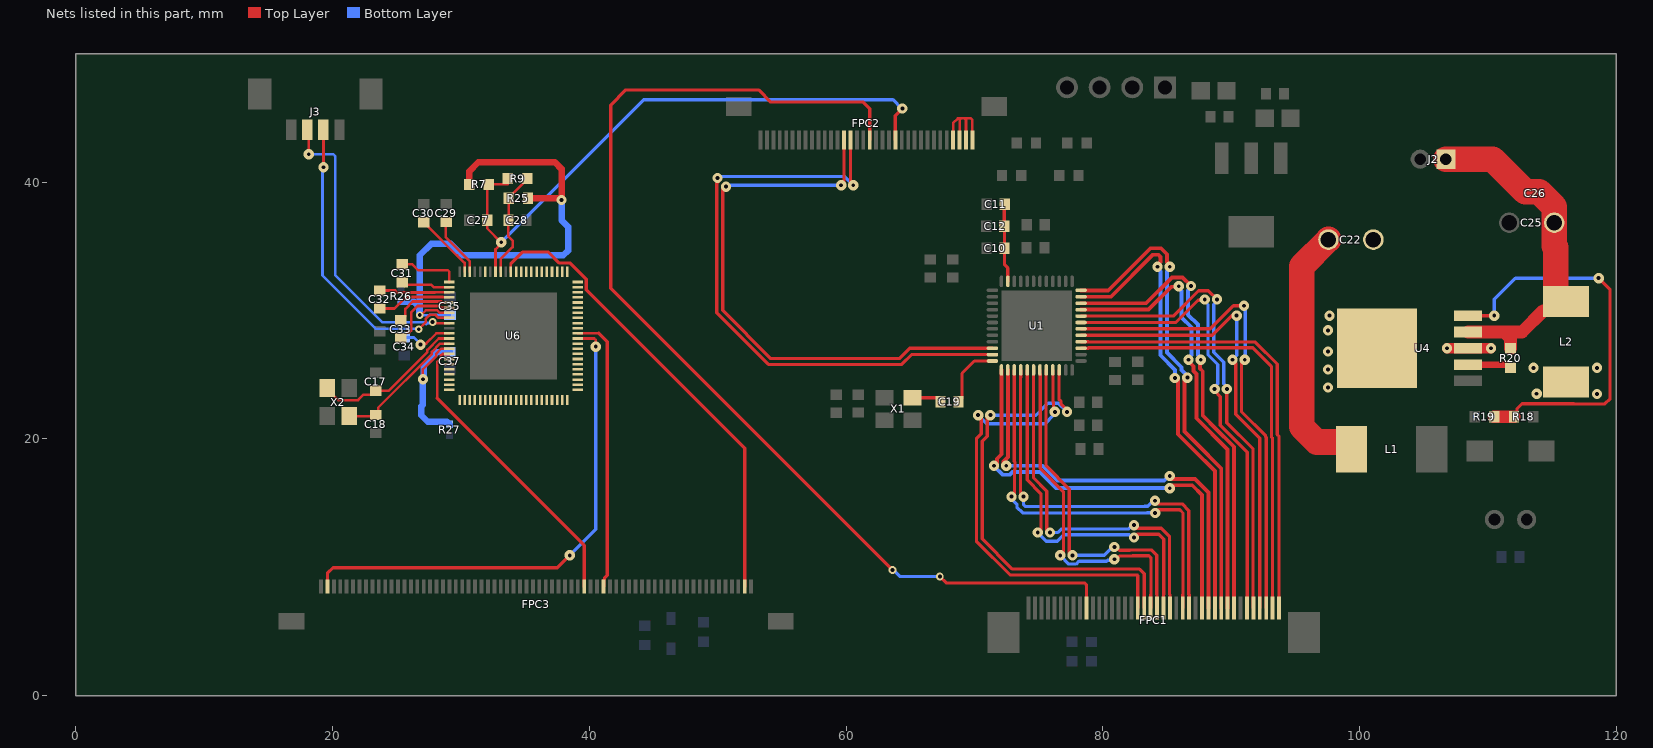
[diagram p0: the nets of this part, all layers, seen from the top]
# Altium PCB MISC71201-3.PcbDoc (part 3 of 3)
Units mm, origin at the board's own origin, x right, y up, seen from the top; angles counter-clockwise.
Board outline 120 x 50 mm, 4 copper layers (Top Layer, Layer 1, Layer 2, Bottom Layer), stack 0.603 mm thick; 69 components, 139 nets, 430 pads, 271 vias.

## Via types
v1: diameter 0.8, hole 0.3, Top Layer to Bottom Layer, 182 vias
v2: diameter 0.6, hole 0.3, Top Layer to Bottom Layer, 89 vias

## Nets (pads, with @x,y where several pads share a name; then routed paths per layer and width w, separated by ;. In a path a pad name is that pad's centre, name@x,y a point inside that pad or via, vN(x,y) a via of type N, cw(c..) or ccw(c..) an arc to the next point about the centre after c; other vN are vias at no path point) (continued)
MIPI_TD3_N: FPC2.15 U1.23 | length 48.6
  Top Layer w0.254: v1(49.986,40.311) 50.098,40.199 50.098,40.072 49.943,39.917 49.943,29.809 53.956,25.796 64.337,25.796 65.102,26.561 U1.23@71.407,26.561 ; FPC2.15@60.345,43.277 60.344,42.4 60.344,39.976 v1(60.57,39.751)
  Bottom Layer w0.254: v1(49.986,40.311) 50.103,40.428 59.9,40.428 60.57,39.758 v1(60.57,39.751)
MIPI_TD3_P: FPC2.14 U1.22 | length 45.6
  Top Layer w0.254: v1(50.658,39.639) 50.546,39.751 50.419,39.751 50.397,39.729 50.397,29.997 54.144,26.25 64.149,26.25 64.961,27.061 U1.22@71.407,27.061 ; v1(59.62,39.751) 59.844,39.975 59.844,42.4 FPC2.14@59.845,43.277
  Bottom Layer w0.254: v1(50.658,39.639) 50.77,39.751 v1(59.62,39.751)
NetC10_2: C10.2 C11.2 C12.1 U1.11 | length 6.2
  Top Layer w0.254: C11.2@72.367,38.28 72.319,38.232 C12.1@72.319,36.546 72.337,36.528 C10.2@72.337,34.851 72.337,33.581 72.606,33.312 U1.11@72.606,32.261
NetC19_1: C19.1 U1.24 | length 5.1
  Top Layer w0.254: C19.1@68.763,22.893 69.036,23.166 69.036,25.094 70.003,26.061 U1.24@71.407,26.061
NetC19_2: C19.2 X1.3 | length 2.3
  Top Layer w0.254: X1.3@65.184,23.208 67.09,23.208 67.363,22.935 C19.2@67.363,22.893
NetC22_1: C22.1 L2.1 U4.3 U4.6 | length 3.4
  Top Layer w0.8: v1(106.807,27.051) U4.3@108.445,27.051 v1(110.236,27.051)
  other v1: 118.491,23.495 113.792,23.514 97.536,24.003 97.536,25.4 113.538,25.527 118.491,25.527 97.536,26.797 97.536,28.448 97.663,29.591
NetC22_2: C22.2 L1.1 | length 20.2
  Top Layer w2: C22.2@97.575,35.519 95.504,33.448 95.504,20.928 96.676,19.756 99.149,19.756 99.361,19.544 L1.1@99.361,19.177
NetC31_1: C31.1 U6.1 | length 4.7
  Top Layer w0.2: C31.1@25.446,33.599 26.208,33.599 26.678,33.129 28.984,33.129 29.101,33.012 U6.1@29.101,32.215
NetC31_2: C31.2 U6.2 | length 3.8
  Top Layer w0.2: C31.2@25.446,32.2 25.641,32.004 27.686,32.004 27.875,31.815 U6.2@29.101,31.815
NetC32_1: C32.1 U6.3 | length 5.5
  Top Layer w0.2: C32.1@23.675,31.552 24.89,31.552 25.045,31.397 27.968,31.397 27.986,31.415 U6.3@29.101,31.415
NetC32_2: C32.2 U6.4 | length 5.8
  Top Layer w0.2: C32.2@23.675,30.152 24.818,30.152 25.713,31.047 28.612,31.047 28.644,31.015 U6.4@29.101,31.015
NetC33_1: C33.1 U6.5 | length 4.7
  Top Layer w0.2: C33.1@25.326,29.251 25.376,29.251 25.676,29.551 25.676,30.121 26.252,30.697 28.467,30.697 28.549,30.615 U6.5@29.101,30.615
NetC33_2: C33.2 U6.6 | length 5.7
  Top Layer w0.2: C33.2@25.326,27.851 25.376,27.851 25.829,28.304 26.006,28.304 26.147,28.446 26.147,29.86 26.634,30.347 28.322,30.347 28.454,30.215 U6.6@29.101,30.215
NetR18_1: R18.1 R19.1 U4.5 | length 31.7
  Top Layer w0.254: U4.5@108.445,29.591 v1(110.49,29.591) ; R18.1@112.024,21.717 112.262,21.955 112.262,22.346 112.649,22.733 116.675,22.733 116.694,22.714 119.107,22.714 119.507,23.114 119.507,31.623 v1(118.618,32.512)
  Top Layer w1: R19.1@110.48,21.717 R18.1@112.024,21.717
  Bottom Layer w0.254: v1(110.49,29.591) 110.49,30.861 112.141,32.512 v1(118.618,32.512)
NetR20_1: R20.1 U4.2 | length 3.4
  Top Layer w0.254: R20.1@111.516,25.781 R20.1@111.76,25.537
  Top Layer w0.5: U4.2@108.445,25.781 R20.1@111.516,25.781
PWM: FPC1.10 FPC2.18 | length 86.4
  Top Layer w0.254: FPC2.18@61.845,43.277 61.845,45.724 61.341,46.228 54.133,46.228 53.189,47.173 42.855,47.173 41.67,45.988 41.67,31.736 v2(63.627,9.779) ; v2(67.31,9.271) 67.804,8.777 78.577,8.777 78.726,8.628 FPC1.10@78.726,6.825
  Bottom Layer w0.254: v2(63.627,9.779) 63.706,9.779 64.214,9.271 v2(67.31,9.271)
RESET#: C27.1 FPC2.22 R7.1 R9.2 U6.81 | length 48.2
  Top Layer w0.2: U6.81@32.701,33.015 32.701,34.762 33.147,35.208 v1(33.147,35.306) 32.06,36.393 C27.1@32.06,37.031 32.06,39.707 R7.1@32.171,39.818 33.663,39.818 R9.2@33.663,40.259
  Top Layer w0.254: FPC2.22@63.845,43.277 63.845,45.16 64.389,45.704 v1(64.389,45.72)
  Bottom Layer w0.254: v1(33.147,35.306) 44.243,46.402 63.666,46.402 64.348,45.72 v1(64.389,45.72)
RFU_NC: FPC2.31 FPC2.32 FPC2.33 FPC2.34 | length 8
  Top Layer w0.2: FPC2.31@68.345,43.277 68.345,44.596 68.707,44.958 68.962,44.958 ; FPC2.32@68.845,43.277 68.845,44.841 68.962,44.958 ; FPC2.33@69.345,43.277 69.345,44.83 69.217,44.958 ; FPC2.34@69.845,43.277 69.845,44.841 69.728,44.958 69.217,44.958 ; 68.962,44.958 69.217,44.958
RX1: FPC3.42 U6.15 | length 23.6
  Top Layer w0.21: 28.154,23.154 28.154,25.995 28.446,26.287 28.446,26.487 28.569,26.61 29.096,26.61 U6.15@29.101,26.615
  Top Layer w0.254: 28.154,23.154 39.61,11.698 FPC3.42@39.61,8.484
RX2: U6.16
RX3: U6.17
RX4: U6.18
RX5: U6.19
RX6: U6.20
RX7: U6.21
RX8: U6.22
RX9: U6.23
RX10: U6.24
RX11: U6.25
RX12: U6.26
RX13: U6.27
RX14: U6.28
RX15: U6.29
RX16: U6.30
RX17: U6.31
RX18: U6.32
RX19: U6.33
RX20: U6.34
RX21: U6.35
RX22: U6.36
RX23: U6.37
RX24: U6.38
RX25: U6.39
RX26: U6.40
RX27: U6.41
RX28: U6.42
RX29: U6.43
RX30: U6.44
RX31: U6.45
RX32: U6.46
RX33: U6.47
RX34: U6.48
RX35: U6.49
RX36: U6.50
RX37: U6.51
RX38: U6.52
RX39: U6.53
RX40: U6.54
RX41: FPC3.2 U6.55 | length 39.6
  Top Layer w0.2: U6.55@39.101,27.815 40.384,27.815 40.513,27.686 v1(40.513,27.178)
  Top Layer w0.254: FPC3.2@19.61,8.484 19.61,9.525 20.043,9.958 37.517,9.958 v1(38.481,10.922)
  Bottom Layer w0.254: v1(38.481,10.922) 40.513,12.954 v1(40.513,27.178)
RXE0_N: FPC1.30 U1.47 | length 36.9
  Top Layer w0.3: U1.47@78.306,31.062 80.633,31.062 83.913,34.342 84.316,34.342 84.492,34.166 84.492,33.761 84.267,33.536 v1(84.267,33.401) ; v1(85.615,24.745) 85.655,24.745 85.86,24.54 85.86,20.359 87.042,19.177 88.726,17.493 88.726,7.875 FPC1.30@88.726,6.825
  Bottom Layer w0.3: v1(84.267,33.401) 84.267,33.266 84.492,33.041 84.492,26.504 85.632,25.364 85.632,24.762 v1(85.615,24.745)
RXE0_P: FPC1.31 U1.48 | length 37.9
  Top Layer w0.3: U1.48@78.306,31.562 80.426,31.562 83.706,34.842 84.523,34.842 84.992,34.373 84.992,33.761 85.217,33.536 v1(85.217,33.401) ; v1(86.585,24.765) 86.36,24.54 86.36,20.566 87.249,19.677 89.226,17.7 89.226,7.875 FPC1.31@89.226,6.825
  Bottom Layer w0.3: v1(85.217,33.401) 85.217,33.266 84.992,33.041 84.992,26.712 86.132,25.571 86.132,25.353 86.585,24.9 v1(86.585,24.765)
RXE1_N: FPC1.32 U1.45 | length 35.2
  Top Layer w0.3: U1.45@78.306,30.061 83.574,30.061 85.353,31.84 85.881,31.84 v1(85.918,31.877) ; v1(86.68,26.162) 86.68,26.027 87.059,25.648 87.059,25.281 87.285,25.055 87.285,21.607 89.726,19.166 FPC1.32@89.726,6.825
  Bottom Layer w0.3: v1(85.918,31.877) 85.918,31.742 86.143,31.517 86.143,29.451 86.905,28.689 86.905,26.522 86.68,26.297 v1(86.68,26.162)
RXE1_P: FPC1.33 U1.46 | length 36.4
  Top Layer w0.3: U1.46@78.306,30.562 83.367,30.561 85.383,32.577 86.208,32.577 86.868,31.917 v1(86.868,31.907) ; v1(87.63,26.162) 87.559,26.091 87.559,25.488 87.785,25.262 87.785,21.814 88.9,20.699 90.079,19.52 90.226,19.373 FPC1.33@90.226,6.825
  Bottom Layer w0.3: v1(86.868,31.907) 86.868,31.771 86.643,31.546 86.643,29.658 87.405,28.896 87.405,26.522 87.63,26.297 v1(87.63,26.162)
RXE2_N: FPC1.35 U1.43 | length 36
  Top Layer w0.254: U1.43@78.306,29.06 85.687,29.06 87.417,30.79 87.879,30.79 v1(87.946,30.857) ; v1(88.712,23.876) 88.712,23.728 89.154,23.286 89.154,21.049 91.249,18.954 91.249,6.848 FPC1.35@91.226,6.825
  Bottom Layer w0.254: v1(87.946,30.857) 87.946,30.71 88.196,30.46 88.196,26.553 88.96,25.789 88.96,24.272 88.712,24.024 v1(88.712,23.876)
RXE2_P: FPC1.36 U1.44 | length 37.1
  Top Layer w0.254: U1.44@78.306,29.561 85.48,29.561 87.453,31.534 88.227,31.534 v1(88.9,30.861) ; v1(89.662,23.876) 89.662,21.248 91.703,19.207 91.703,6.848 FPC1.36@91.726,6.825
  Bottom Layer w0.254: v1(88.9,30.861) 88.9,30.713 88.65,30.463 88.65,26.741 89.414,25.977 89.414,24.272 89.662,24.024 v1(89.662,23.876)
RXE3_N: FPC1.39 U1.39 | length 34.3
  Top Layer w0.254: U1.39@78.306,27.061 78.883,27.061 78.906,27.085 91.694,27.085 93.138,25.641 93.138,20.143 93.226,20.055 FPC1.39@93.226,6.825
RXE3_P: FPC1.40 U1.40 | length 35.1
  Top Layer w0.254: U1.40@78.306,27.562 78.883,27.562 78.906,27.539 91.882,27.539 93.592,25.829 93.592,20.331 93.726,20.197 FPC1.40@93.726,6.825
RXEC_N: FPC1.37 U1.41 | length 36.7
  Top Layer w0.254: U1.41@78.306,28.062 88.521,28.062 90.237,29.778 v1(90.424,29.591) ; v1(90.103,26.162) 90.351,25.914 90.351,21.917 92.226,20.042 FPC1.37@92.226,6.825
  Bottom Layer w0.254: v1(90.103,26.162) 90.103,26.169 90.424,26.49 v1(90.424,29.591)
RXEC_P: FPC1.38 U1.42 | length 37.9
  Top Layer w0.254: U1.42@78.306,28.563 88.38,28.563 90.175,30.358 v1(91,30.358) ; v1(91.053,26.162) 90.805,25.914 90.805,22.105 92.68,20.23 92.68,20.153 92.726,20.107 FPC1.38@92.726,6.825
  Bottom Layer w0.254: v1(91,30.358) 91.101,30.258 91.101,26.21 v1(91.053,26.162)
RXO0_N: FPC1.18 U1.33 | length 36.4
  Top Layer w0.254: v1(70.291,21.844) 70.412,21.844 70.539,21.717 70.539,20.381 70.158,20 70.158,12.012 72.772,9.398 82.677,9.398 82.726,9.349 FPC1.18@82.726,6.825 ; U1.33@76.106,25.362 76.106,25.045 76.13,25.022 76.13,22.89 76.162,22.858 76.162,22.202 v1(76.266,22.098)
  Bottom Layer w0.254: v1(70.291,21.844) 70.291,21.837 70.961,21.167 75.523,21.167 75.802,21.446 75.802,21.487 76.266,21.95 v1(76.266,22.098)
RXO0_P: FPC1.19 U1.34 | length 36.6
  Top Layer w0.254: v1(71.241,21.844) 71.12,21.844 70.993,21.717 70.993,20.193 70.612,19.812 70.612,12.2 72.96,9.852 82.865,9.852 83.226,9.491 FPC1.19@83.226,6.825 ; U1.34@76.607,25.362 76.607,25.045 76.584,25.022 76.584,23.078 76.752,22.909 76.752,22.709 77.216,22.246 v1(77.216,22.098)
  Bottom Layer w0.254: v1(71.241,21.844) 74.797,21.844 75.728,22.775 76.546,22.775 77.216,22.105 v1(77.216,22.098)
RXO1_N: FPC1.20 U1.31 | length 26.9
  Top Layer w0.254: U1.31@75.106,25.362 75.106,25.045 75.129,25.022 75.129,17.701 76.935,15.895 76.935,11.106 76.751,10.922 v1(76.687,10.922) ; v1(80.899,10.619) 81.047,10.619 81.295,10.867 82.292,10.867 82.317,10.892 83.6,10.892 83.749,10.743 83.749,7.875 83.726,7.852 FPC1.20@83.726,6.825
  Bottom Layer w0.254: v1(76.687,10.922) 76.687,10.915 77.357,10.245 77.918,10.245 78.141,10.468 80.292,10.468 80.373,10.549 80.829,10.549 v1(80.899,10.619)
RXO1_P: FPC1.21 U1.32 | length 26.6
  Top Layer w0.254: U1.32@75.606,25.362 75.606,25.045 75.583,25.022 75.583,17.889 77.389,16.083 77.389,11.106 77.573,10.922 v1(77.637,10.922) ; v1(80.899,11.569) 81.047,11.569 81.295,11.321 82.104,11.321 82.129,11.346 83.788,11.346 84.203,10.931 84.203,7.875 84.226,7.852 FPC1.21@84.226,6.825
  Bottom Layer w0.254: v1(77.637,10.922) 80.104,10.922 80.751,11.569 v1(80.899,11.569)
RXO2_N: FPC1.22 U1.29 | length 29.3
  Top Layer w0.254: U1.29@74.107,25.362 74.107,16.808 75.184,15.732 75.184,12.827 75.057,12.7 v1(74.936,12.7) ; v1(82.427,12.321) 82.427,12.329 82.671,12.573 84.368,12.573 84.749,12.192 84.749,7.875 84.726,7.852 FPC1.22@84.726,6.825
  Bottom Layer w0.254: v1(74.936,12.7) 74.936,12.693 75.606,12.023 76.445,12.023 76.941,12.519 82.081,12.519 82.279,12.321 v1(82.427,12.321)
RXO2_P: FPC1.23 U1.30 | length 28.8
  Top Layer w0.254: U1.30@74.608,25.362 74.608,16.95 75.638,15.92 75.638,12.827 75.765,12.7 v1(75.886,12.7) ; v1(82.423,13.275) 82.671,13.027 84.556,13.027 85.203,12.38 85.203,7.875 85.226,7.852 FPC1.23@85.226,6.825
  Bottom Layer w0.254: v1(75.886,12.7) 75.887,12.701 76.481,12.701 76.753,12.973 81.973,12.973 82.275,13.275 v1(82.423,13.275)
RXO3_N: FPC1.28 U1.25 | length 34.1
  Top Layer w0.3: v1(71.53,17.907) 71.628,17.907 71.755,18.034 71.755,18.445 72.106,18.796 72.106,24.762 U1.25@72.106,25.362 ; v1(85.219,16.155) 85.219,16.16 85.442,16.383 86.964,16.383 87.726,15.621 87.726,7.875 FPC1.28@87.726,6.825
  Bottom Layer w0.3: v1(71.53,17.907) 71.53,17.867 72.19,17.207 72.77,17.207 72.97,17.407 75.104,17.407 76.353,16.158 85.216,16.158 v1(85.219,16.155)
RXO3_P: FPC1.29 U1.26 | length 33.6
  Top Layer w0.3: v1(72.48,17.907) 72.382,17.907 72.255,18.034 72.255,18.238 72.606,18.589 72.606,24.762 U1.26@72.606,25.362 ; v1(85.217,17.108) 85.442,16.883 87.171,16.883 88.226,15.828 88.226,7.875 FPC1.29@88.226,6.825
  Bottom Layer w0.3: v1(72.48,17.907) 75.311,17.907 76.454,16.764 84.791,16.764 85.135,17.108 v1(85.217,17.108)
RXOC_N: FPC1.25 U1.27 | length 31.8
  Top Layer w0.254: v1(72.882,15.494) 73.003,15.494 73.13,15.621 73.13,17.599 73.157,17.627 73.157,18.187 73.107,18.238 U1.27@73.107,25.362 ; v1(84.077,14.227) 84.077,14.233 84.322,14.478 85.995,14.478 86.249,14.224 86.249,7.875 86.226,7.852 FPC1.25@86.226,6.825
  Bottom Layer w0.254: v1(72.882,15.494) 72.882,15.346 73.315,14.913 73.315,14.675 73.76,14.23 83.448,14.23 83.463,14.245 84.059,14.245 v1(84.077,14.227)
RXOC_P: FPC1.26 U1.28 | length 31.7
  Top Layer w0.254: U1.28@73.607,25.362 73.607,24.785 73.584,24.762 73.584,15.621 73.711,15.494 v1(73.832,15.494) ; v1(84.074,15.18) 84.322,14.932 86.183,14.932 86.703,14.412 86.703,7.875 86.726,7.852 FPC1.26@86.726,6.825 ; FPC1.26@86.73,6.829 FPC1.26@86.734,6.825
  Bottom Layer w0.254: v1(73.832,15.494) 73.817,15.479 73.817,14.883 73.968,14.732 83.24,14.732 83.255,14.747 83.493,14.747 83.926,15.18 v1(84.074,15.18)
TX1: FPC3.67 U6.78 | length 36.8
  Top Layer w0.2: U6.78@33.901,33.015 33.901,33.647
  Top Layer w0.254: 33.901,33.647 34.798,34.544 36.83,34.544 37.682,33.692 38.516,33.692 39.778,32.429 39.778,31.596 52.11,19.264 FPC3.67@52.11,8.484
TX2: U6.77
TX3: U6.76
TX4: U6.75
TX5: U6.74
TX6: U6.73
TX7: U6.72
TX8: U6.71
TX9: U6.70
TX10: U6.69
TX11: U6.68
TX12: U6.67
TX13: U6.66
TX14: U6.65
TX15: U6.64
TX16: U6.63
TX17: U6.62
TX18: U6.61
TX19: U6.60
TX20: U6.59
TX21: U6.58
TX22: U6.57
TX23: FPC3.45 U6.56 | length 21.8
  Top Layer w0.2: U6.56@39.101,28.215 40.746,28.215
  Top Layer w0.254: 40.746,28.215 41.402,27.559 41.402,9.368 41.183,9.149 41.183,9.056 41.133,9.006 41.133,8.507 FPC3.45@41.11,8.484
TXD: U6.83
USB_D+: J3.3 U6.9 | length 23.9
  Top Layer w0.2: J3.3@18.044,44.066 18.161,43.949 v1(18.161,42.164) ; v2(27.804,29.097) 27.912,29.097 27.994,29.015 U6.9@29.101,29.015
  Bottom Layer w0.2: v1(18.161,42.164) 20.066,42.164 20.211,42.019 20.211,32.748 23.876,29.083 27.164,29.083 27.306,28.941 27.385,29.02 27.727,29.02 v2(27.804,29.097)
USB_D-: J3.2 U6.8 | length 23.7
  Top Layer w0.2: J3.2@19.294,44.066 19.304,44.056 v1(19.304,41.148) ; v2(26.72,28.533) 27.254,29.067 27.254,29.325 27.576,29.647 28.032,29.647 28.264,29.415 U6.8@29.101,29.415
  Bottom Layer w0.2: v1(19.304,41.148) 19.226,41.07 19.226,32.717 23.368,28.575 26.678,28.575 v2(26.72,28.533)
VDD3A: C37.2 R27.2 U6.14 | length 12.5
  Top Layer w0.2: v1(27.051,24.638) 27.051,25.418 28.091,26.458 28.091,26.634 28.472,27.015 U6.14@29.101,27.015
  Bottom Layer w0.5: R27.2@29.134,21.128 29.134,21.14 29.113,21.161 29.101,21.161 28.926,21.336 27.432,21.336 26.924,21.844 26.924,22.541 27.051,22.668 v1(27.051,24.638) 27.108,24.695 27.108,25.711 28.156,26.759 C37.2@29.136,26.759
VDD3D: C35.2 R7.2 R25.2 R26.2 U6.7 | length 42.2
  Top Layer w0.2: v2(26.797,29.633) 26.905,29.633 27.269,29.997 28.177,29.997 28.359,29.815 U6.7@29.101,29.815
  Top Layer w0.5: R7.2@30.664,39.818 30.664,40.824 31.369,41.529 37.338,41.529 37.846,41.021 v1(37.846,38.608) 37.765,38.608 37.635,38.738 R25.2@35.232,38.738
  Bottom Layer w0.2: v2(26.797,29.633) 27.562,29.633 27.576,29.647 28.185,29.647 28.198,29.633 29.145,29.633 C35.2@29.157,29.644
  Bottom Layer w0.5: R26.2@25.342,30.688 26.335,30.688 26.778,30.245 26.778,29.652 v2(26.797,29.633) 26.797,34.29 27.686,35.179 29.21,35.179 30.099,34.29 37.986,34.29 38.354,34.658 38.354,36.525 37.846,37.033 v1(37.846,38.608)
VDD16: C34.2 U6.11 | length 4.1
  Top Layer w0.2: v1(26.859,27.333) 26.946,27.42 27.293,27.42 28.088,28.215 U6.11@29.101,28.215
  Bottom Layer w0.2: 26.342,27.887 26.859,27.37 v1(26.859,27.333)
  Bottom Layer w0.254: C34.2@25.58,27.887 26.342,27.887
VDDIO: C28.2 R9.1 R25.1 U6.80 | length 8.4
  Top Layer w0.2: U6.80@33.101,33.015 33.101,33.99 34.036,34.925 34.036,35.433 33.708,35.761 C28.2@33.708,37.031 33.726,37.048 R25.1@33.726,38.738 34.03,39.069 34.865,39.927 R9.1@35.169,40.259
VGH: C30.2 U6.87 | length 5.2
  Top Layer w0.2: C30.2@27.104,36.868 27.154,36.868 27.454,36.568 27.454,36.519 29.682,34.29 29.718,34.29 30.301,33.707 U6.87@30.301,33.015
VIN: C25.1 C26.2 J2.1 L2.2 R20.2 U4.4 | length 29.5
  Top Layer w1: U4.4@108.445,28.321 111.252,28.321 ; R20.2@111.76,27.043 111.76,27.813 111.252,28.321 ; L2.2@115.366,29.975 114.303,29.975 112.649,28.321 111.252,28.321
  Top Layer w2: J2.1@106.724,41.783 110.363,41.783 112.903,39.243 113.989,39.243 115.161,38.071 C25.1@115.161,36.83 115.161,35.006 115.268,34.899 115.268,30.899 L2.2@115.824,30.899
  Bottom Layer w1: C26.2@114.366,39.116 115.046,38.436 115.046,36.945 C25.1@115.161,36.83
VTX: C29.2 U6.86 | length 4.7
  Top Layer w0.2: C29.2@28.882,36.883 28.829,36.83 28.829,35.687 30.701,33.815 U6.86@30.701,33.015
XT_IN: C17.2 U6.12 X2.3 | length 12
  Top Layer w0.2: X2.3@19.597,23.96 19.597,23.86 20.447,23.01 22.001,23.01 22.436,23.446 23.068,23.446 C17.2@23.368,23.746 24.389,23.746 27.391,26.748 27.391,26.924 28.282,27.815 U6.12@29.101,27.815
XT_OUT: C18.2 U6.13 X2.1 | length 10.5
  Top Layer w0.2: X2.1@21.297,21.76 23.281,21.76 23.568,22.047 23.568,22.43 27.741,26.603 27.741,26.779 28.377,27.415 U6.13@29.101,27.415
pads on no net: FPC1.14 FPC1.15 FPC1.16 FPC1.41 FPC1.42 FPC2.35 FPC2.36 FPC3.3 FPC3.4 FPC3.5 FPC3.6 FPC3.7 FPC3.8 FPC3.9 FPC3.10 FPC3.11 FPC3.12 FPC3.13 FPC3.14 FPC3.15 FPC3.16 FPC3.17 FPC3.18 FPC3.19 FPC3.20 FPC3.21 FPC3.22 FPC3.23 FPC3.24 FPC3.25 FPC3.26 FPC3.27 FPC3.28 FPC3.29 FPC3.30 FPC3.31 FPC3.32 FPC3.33 FPC3.34 FPC3.35 FPC3.36 FPC3.37 FPC3.38 FPC3.39 FPC3.40 FPC3.41 FPC3.46 FPC3.47 FPC3.48 FPC3.49 FPC3.50 FPC3.51 FPC3.52 FPC3.53 FPC3.54 FPC3.55 FPC3.56 FPC3.57 FPC3.58 FPC3.59 FPC3.60 FPC3.61 FPC3.62 FPC3.63 FPC3.64 FPC3.65 FPC3.66 FPC3.69 FPC3.70 J3.5 J3.6 U1.3 U1.4 U1.6 U1.12 X1.1

## Polygon pours and split planes (outlines as drawn)
+3.3V2 on Top Layer "GND" (solid, pour order 12): 93.375,33.257 93.359,33.274 89.789,33.274 88.9,34.163 88.9,37.719 90.856,39.675 90.856,47.041 91.948,48.133 92.837,48.133 93.345,47.625 93.345,44.323 92.202,43.18 92.202,40.259 94.742,37.719 94.742,34.163 93.853,33.274
GND on Top Layer "GND_L01_P007" (solid, pour order 7): 107.061,24.765 107.315,25.019 110.744,25.019 111.379,24.384 112.014,24.384 112.522,23.876 112.522,23.241 112.141,22.86 107.315,22.86 107.061,23.114
+12V on Top Layer "+12V_L01_P006" (solid, pour order 6): 112.649,20.701 113.03,21.082 113.03,22.098 113.284,22.352 116.332,22.352 118.491,20.193 118.491,12.446 117.983,11.938 112.903,11.938 112.141,12.7 112.141,16.637 112.649,17.145 112.649,17.907
GND on Top Layer "GND_L01_P005" (solid, pour order 5): 103.864,16.852 103.886,16.874 103.886,21.336 105.029,22.479 106.553,22.479 106.68,22.606 109.347,22.606 109.601,22.352 109.601,21.082 110.744,19.939 110.744,18.542 111.508,17.778 111.508,12.956 110.744,12.192 105.029,12.192 103.886,13.335
NetC22_1 on Top Layer "NETC22_1_L01_P003" (solid, pour order 3): 96.901,29.718 99.949,32.766 99.949,35.814 101.092,36.957 102.997,36.957 106.045,33.909 106.045,28.067 106.553,27.559 110.34,27.559 110.617,27.282 110.617,26.797 110.363,26.543 106.68,26.543 106.172,26.035 106.172,23.495 105.537,22.86 97.409,22.86 96.901,23.368
NetC22_1 on Top Layer "NETC22_1_L01_P000" (solid, pour order 0): 112.776,23.622 112.776,25.4 113.792,26.416 118.491,26.416 119.126,25.781 119.126,23.241 118.872,22.987 113.411,22.987
NetC22_1 on Bottom Layer "NETC22_1_L04_P004" (solid, pour order 4): 96.901,29.718 98.044,30.861 110.338,30.861 112.522,28.677 112.522,27.178 113.157,26.543 118.237,26.543 119.38,25.4 119.38,22.86 118.999,22.479 97.536,22.479 96.901,23.114
GND on Layer 1 "GND_L02_P008" (solid, pour order 8): 4.572,36.462 11.557,43.447 11.557,46.228 14.351,49.022 104.789,49.022 112.663,41.148 116.713,41.148 119.38,38.481 119.38,12.058 116.466,9.144 112.903,9.144 106.045,2.286 15.367,2.286 8.382,9.271 5.461,9.271 4.572,10.16
"3.3V for Touch&TFT" on Layer 2 "Layer 2-3.3V for Touch&TFT" (solid, pour order 11): 55.742,15.886 68.707,2.921 94.869,2.921 97.549,5.601 97.549,34.785 86.995,45.339 86.995,46.609 85.09,48.514 66.675,48.514 64.135,45.974 64.135,38.608 63.5,37.973 27.051,37.973 22.733,33.655 22.733,19.05 25.897,15.886

## Silkscreen, mask and mechanical layers (free items; w line width, h text height)
Top Overlay:
  circle w0.254: c115,5 r3.5
  circle w0.254: c5,45 r3.5
  circle w0.254: c115,45 r3.5
  circle w0.254: c5,5 r3.5
Mechanical 1:
  circle w0.21: c5,45 r1.75
  circle w0.21: c115,45 r1.75
  circle w0.21: c115,5 r1.75
  circle w0.21: c5,5 r1.75
  lines w0.254: 0,0 120,0 120,50 0,50 0,0